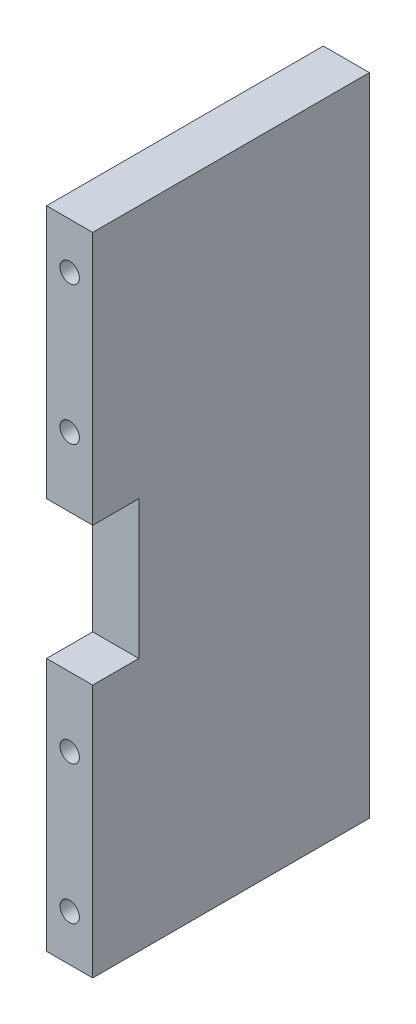
from build123d import *

# Parameters (mm, degrees)
SKETCH_1_W             = 60
SKETCH_1_H             = 140
BOSS_EXTRUDE_1_DEPTH   = 10
SKETCH_4_W             = 10
SKETCH_4_H             = 30
CUT_EXTRUDE_1_DEPTH    = 77.811457479
LINEAR_PATTERN_2_COUNT = 3
LINEAR_PATTERN_2_PITCH = 60
M5_TAPPED_HOLE_3_D     = 4.2
M5_TAPPED_HOLE_3_DEPTH = 12.4
M5_TAPPED_HOLE_3_TIP   = 1.2618073


with BuildPart() as part:
    # Sketch 1 → Boss-Extrude 1 (new body)
    with BuildSketch(Plane(origin=(0, 0, 0), x_dir=(0, 0, -1), z_dir=(1, 0, 0))):
        Rectangle(SKETCH_1_W, SKETCH_1_H)
    extrude(amount=BOSS_EXTRUDE_1_DEPTH)

    # Sketch 4 → Cut-Extrude 1 (cut, through all)
    with BuildSketch(Plane.ZY):
        with Locations((25, 0)):
            Rectangle(SKETCH_4_W, SKETCH_4_H)
    extrude(amount=-CUT_EXTRUDE_1_DEPTH, mode=Mode.SUBTRACT)

    # Sketch 5 → M5 Tapped Hole 2 (revolve, cut)
    with BuildSketch(Plane(origin=(5, 60, -30), x_dir=(0, 1, 0), z_dir=(1, 0, 0))):
        Polygon((0, 0), (0, 13.6618073), (2.1, 12.4), (2.1, 0), align=None)
    m5_tapped_hole_2 = revolve(axis=Axis((5, 60, -36.35), (0, 0, 1)), mode=Mode.SUBTRACT)

    # Linear Pattern 2: M5 Tapped Hole 2 ×3
    with Locations(*[(0, -i * LINEAR_PATTERN_2_PITCH, 0) for i in range(1, LINEAR_PATTERN_2_COUNT)]):
        add(m5_tapped_hole_2, mode=Mode.SUBTRACT)

    # M5 Tapped Hole 3
    with Locations(Plane.XY.offset(30)):
        with Locations((5, -60), (5, -30), (5, 30), (5, 60)):
            Hole(M5_TAPPED_HOLE_3_D / 2, depth=M5_TAPPED_HOLE_3_DEPTH)
            with Locations((0, 0, -(M5_TAPPED_HOLE_3_DEPTH + M5_TAPPED_HOLE_3_TIP / 2))):  # 118° drill point
                Cone(0, M5_TAPPED_HOLE_3_D / 2, M5_TAPPED_HOLE_3_TIP, mode=Mode.SUBTRACT)


solid = part.part
